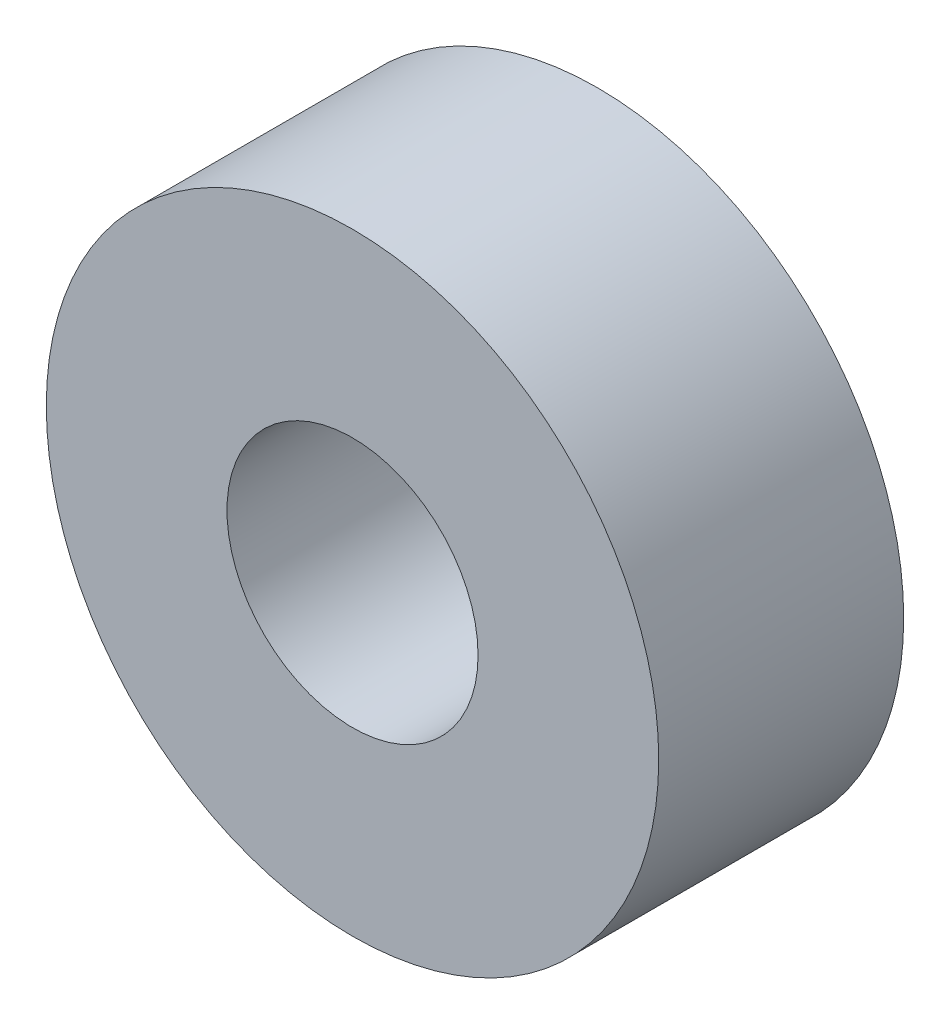
from build123d import *

# Parameters (mm, degrees)
SKETCH_1_R      = 20
SKETCH_1_R_2    = 8.2
EXTRUDE_1_DEPTH = 8


with BuildPart() as part:
    # 草图1 → 凸台-拉伸1 (new, symmetric)
    with BuildSketch(Plane.XY):
        Circle(SKETCH_1_R)
        Circle(SKETCH_1_R_2, mode=Mode.SUBTRACT)
    extrude(amount=EXTRUDE_1_DEPTH, both=True)


solid = part.part
